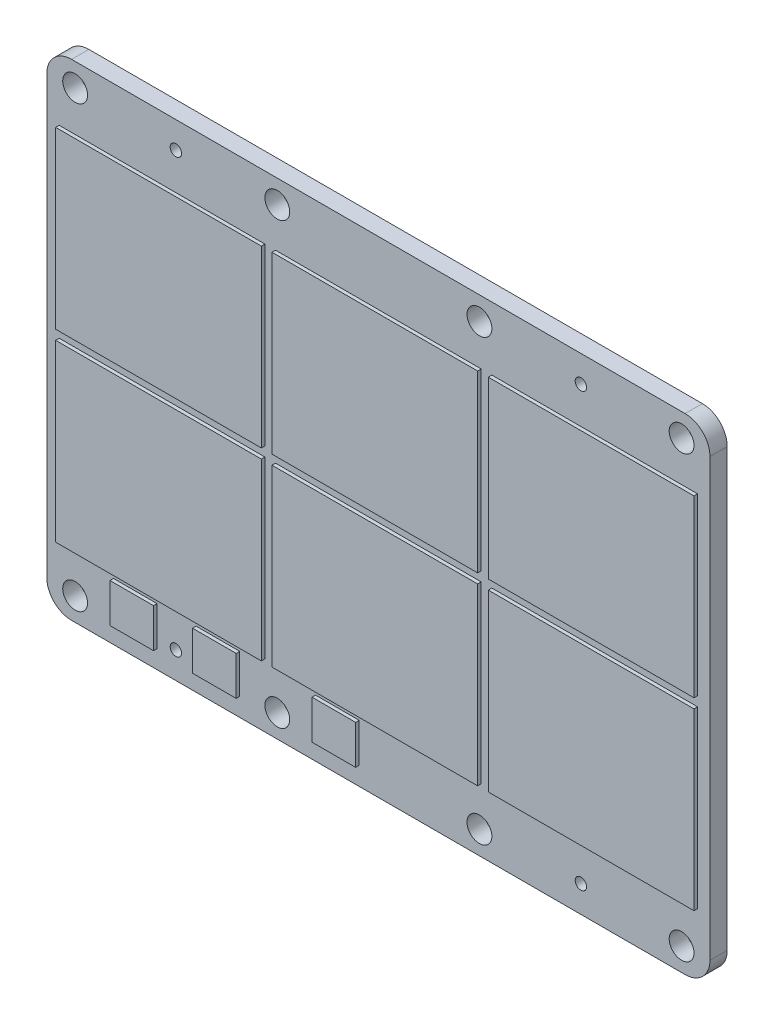
from build123d import *

# Parameters (mm, degrees)
SKETCH1_W                  = 187
SKETCH1_H                  = 137
BOSS_EXTRUDE1_DEPTH        = 4.87
F_7_0_7_DIAMETER_HOLE1_D   = 7
F_3_2_3_2_DIAMETER_HOLE1_D = 3.2
SKETCH6_W                  = 58
SKETCH6_H                  = 101.3
BOSS_EXTRUDE2_DEPTH        = 1
SKETCH7_W                  = 12.3
SKETCH7_H                  = 11
BOSS_EXTRUDE3_DEPTH        = 1
SKETCH8_W                  = 203.41830683
SKETCH8_H                  = 2.7
CUT_EXTRUDE1_DEPTH         = 1
FILLET1_R                  = 7


with BuildPart() as part:
    # Sketch1 → Boss-Extrude1 (new body)
    with BuildSketch(Plane.XY):
        Rectangle(SKETCH1_W, SKETCH1_H)
    extrude(amount=BOSS_EXTRUDE1_DEPTH)

    # Ø7.0 (7) Diameter Hole1 (through all)
    with Locations(Plane.XY.offset(4.87)):
        with Locations((-28.5, 62), (-85.5, 62), (28.5, 62), (85.5, 62), (85.5, -62), (28.5, -62), (-85.5, -62), (-28.5, -62)):
            Hole(F_7_0_7_DIAMETER_HOLE1_D / 2)

    # Ø3.2 (3.2) Diameter Hole1 (through all)
    with Locations(Plane.XY.offset(4.87)):
        with Locations((-57.1, 61.02), (57.1, 60.975), (57.1, -60.975), (-57.1, -61.02)):
            Hole(F_3_2_3_2_DIAMETER_HOLE1_D / 2)

    # Sketch6 → Boss-Extrude2 (add)
    with BuildSketch(Plane.XY.offset(4.87)):
        with Locations((-61, 0)):
            Rectangle(SKETCH6_W, SKETCH6_H)
        Rectangle(SKETCH6_W, SKETCH6_H)
        with Locations((61, 0)):
            Rectangle(SKETCH6_W, SKETCH6_H)
    extrude(amount=BOSS_EXTRUDE2_DEPTH)

    # Sketch7 → Boss-Extrude3 (add)
    with BuildSketch(Plane.XY.offset(4.87)):
        with Locations((-68.55, -57.85)):
            Rectangle(SKETCH7_W, SKETCH7_H)
        with Locations((-45.24, -57.85)):
            Rectangle(SKETCH7_W, SKETCH7_H)
        with Locations((-11.54, -57.85)):
            Rectangle(SKETCH7_W, SKETCH7_H)
    extrude(amount=BOSS_EXTRUDE3_DEPTH)

    # Sketch8 → Cut-Extrude1 (cut)
    with BuildSketch(Plane.XY.offset(5.87)):
        Rectangle(SKETCH8_W, SKETCH8_H)
    extrude(amount=-CUT_EXTRUDE1_DEPTH, mode=Mode.SUBTRACT)

    # Fillet1
    fillet1_edges = [part.edges().sort_by_distance(p)[0] for p in [
        (93.5, -68.5, 2.435),
        (-93.5, -68.5, 2.435),
        (-93.5, 68.5, 2.435),
        (93.5, 68.5, 2.435),
    ]]
    fillet(fillet1_edges, radius=FILLET1_R)


solid = part.part
